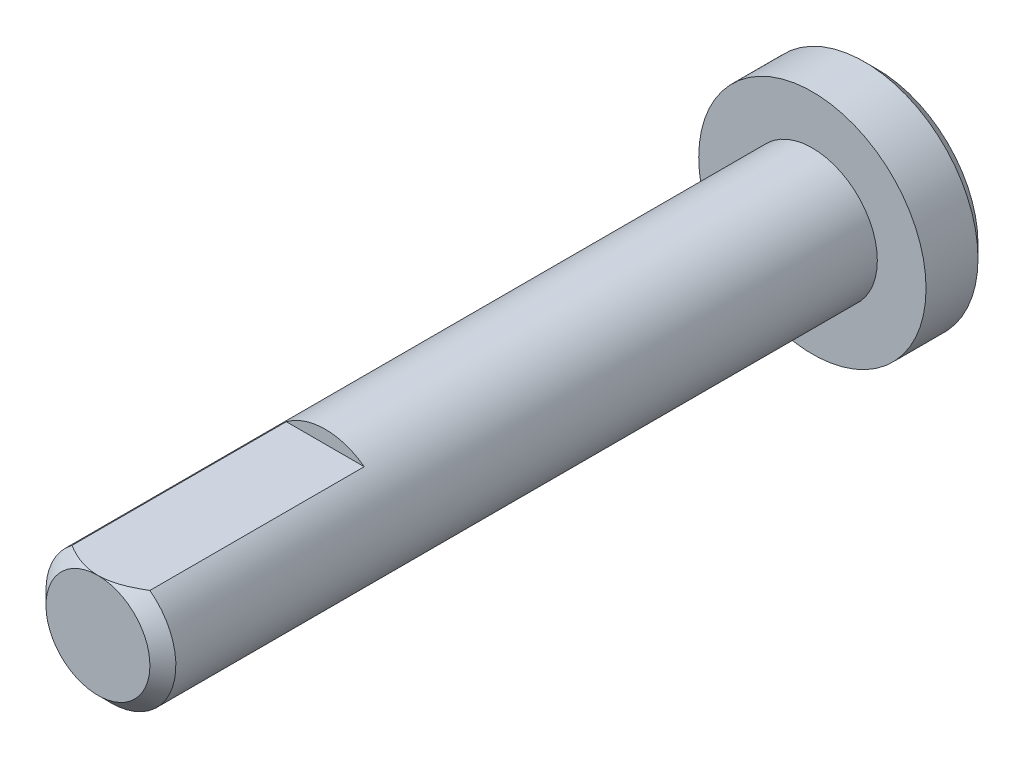
SolidWorks part; units mm, degrees
ref_plane "Front Plane" through (0, 0, 0) normal (0, 0, 1) x (1, 0, 0)
ref_plane "Top Plane" through (0, 0, 0) normal (0, 1, 0) x (1, 0, 0)
ref_plane "Right Plane" through (0, 0, 0) normal (1, 0, 0) x (0, 0, -1)
sketch "Sketch1" plane through (0, 0, 0) normal (0, 0, 1) x (1, 0, 0)
  circle A0 centre (0, 0) radius 1.75
  dimension "D1" = 3.5
extrude "Boss-Extrude1" add sketch "Sketch1" along normal blind 1
sketch "Sketch2" plane through (0, 0, 1) normal (0, 0, 1) x (1, 0, 0)
  circle A0 centre (0, 0) radius 1
  dimension "D1" = 2
extrude "Boss-Extrude2" add sketch "Sketch2" along normal blind 11
chamfer "Chamfer1" distance 0.2 angle 45 2 edges at (1, 0, 12) (1.75, 0, 0)
sketch "Sketch3" plane through (0, 0, 12) normal (0, 0, 1) x (1, 0, 0)
  line L0 (-0.6, 0.8) -> (0.6, 0.8)
  circle A0 centre (0, 0) radius 1 construction
  arc A1 (0.6, 0.8) -> (-0.6, 0.8) centre (0, 0) ccw
  dimension "D1" = 0.8
extrude "Cut-Extrude1" cut sketch "Sketch3" against normal blind 3.5
